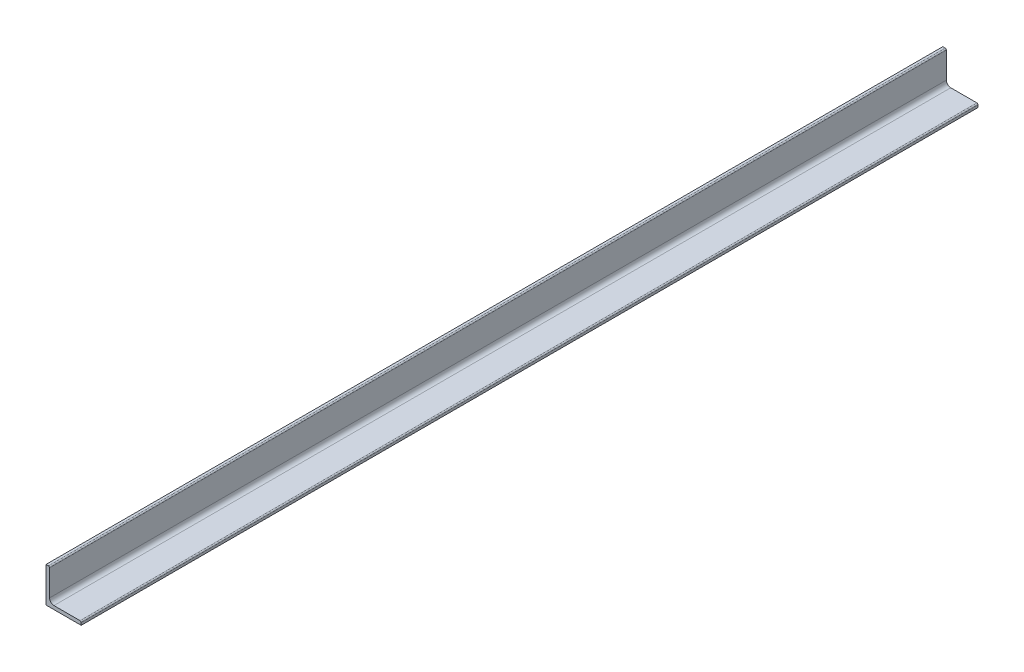
SolidWorks part; units mm, degrees
material "Q235B"
ref_plane "Plane1" through (0, 0, 0) normal (0, 0, 1) x (1, 0, 0)
ref_plane "Plane2" through (0, 0, 0) normal (0, 1, 0) x (1, 0, 0)
ref_plane "Plane3" through (0, 0, 0) normal (1, 0, 0) x (0, 0, -1)
sketch "Sketch1" plane through (0, 0, 0) normal (0, 0, 1) x (1, 0, 0)
  line L0 (0, 0) -> (0, 40)
  line L1 (0, 20) -> (4, 20) construction
  line L2 (4, 38.6667) -> (4, 9)
  line L3 (9, 4) -> (38.6667, 4)
  line L4 (20, 4) -> (20, 0) construction
  line L5 (40, 0) -> (0, 0)
  line L6 (0, 40) -> (2.6667, 40)
  line L7 (40, 0) -> (40, 2.6667)
  arc A0 (40, 2.6667) -> (38.6667, 4) centre (38.6667, 2.6667) ccw
  arc A1 (2.6667, 40) -> (4, 38.6667) centre (2.6667, 38.6667) cw
  arc A2 (9, 4) -> (4, 9) centre (9, 9) cw
  point P10 (20, 0)
  point P14 (0, 20)
  point P15 (4, 20)
  point P16 (20, 4)
  point P17 (4, 40)
  point P18 (40, 4)
  point P21 (40, 4)
  point P24 (4, 40)
extrude "Boss-Extrude1" add sketch "Sketch1" along normal blind 1020 contours L3 A0 L7 L5 L0 L6 A1 L2 A2
equation "\"D2@Sketch1\" = \"D1@Sketch1\" / 3"
